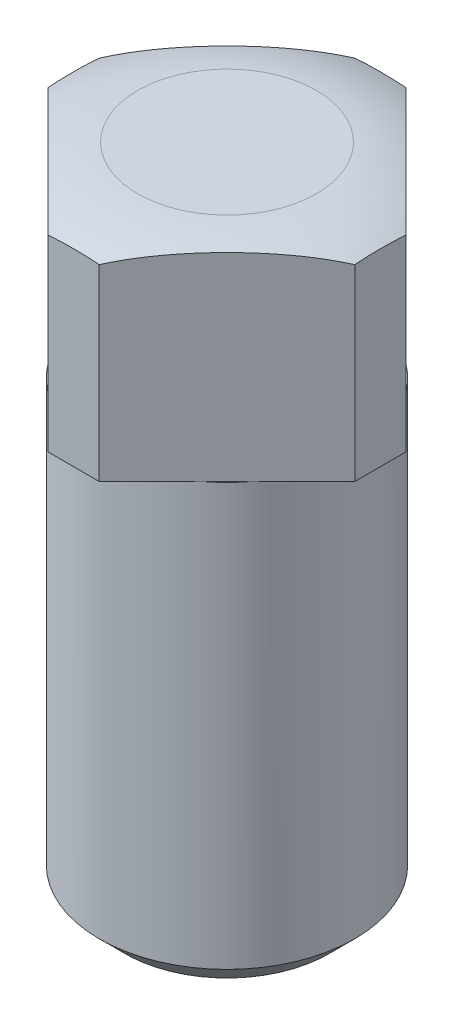
SolidWorks part; units mm, degrees
ref_plane "Front" through (0, 0, 0) normal (0, 0, 1) x (1, 0, 0)
ref_plane "Top" through (0, 0, 0) normal (0, 1, 0) x (1, 0, 0)
ref_plane "Right" through (0, 0, 0) normal (1, 0, 0) x (0, 0, -1)
sketch "Sketch1" plane through (0, 0, 0) normal (0, 0, 1) x (1, 0, 0)
  line L0 (0, 0) -> (0, 24)
  line L1 (0, 24) -> (10, 24)
  line L2 (10, 24) -> (10, 16)
  line L3 (10, 16) -> (5, 16)
  line L4 (5, 16) -> (5, 0)
  line L5 (5, 0) -> (0, 0)
  dimension "D1" = 16
  dimension "D2" = 8
  dimension "D3" = 5
  dimension "D4" = 10
revolve "Revolve1" add sketch "Sketch1" angle 360 about L0
chamfer "Chamfer1" distance 1 angle 45 1 edges at (0, 0, -5)
sketch "Sketch2" plane through (0, 24, 0) normal (0, 1, 0) x (1, 0, 0)
  line L0 (-1, 6) -> (1, 6)
  line L1 (0, 0) -> (0, 8.2576) construction
  line L2 (0, 0) -> (6, 0) construction
  line L3 (-1, -6) -> (1, -6)
  line L4 (6, 1) -> (6, -1)
  line L5 (-6, 1) -> (-6, -1)
  line L6 (-1, 6) -> (-6, 1)
  line L7 (6, 1) -> (1, 6)
  line L9 (6, -1) -> (1, -6)
  line L10 (-1, -6) -> (-6, -1)
  circle A0 centre (0, 0) radius 11.9782
  dimension "D1" = 6
  dimension "D2" = 2
  dimension "D3" = 1
  dimension "D4" = 2
  dimension "D5" = 1
  dimension "D6" = 6
extrude "Cut-Extrude2" cut sketch "Sketch2" against normal up to surface (8 mm away) up to face at (0, 16, -10)
sketch "Sketch3" plane through (0, 0, 0) normal (0, 0, 1) x (1, 0, 0)
  line L0 (3.5, 24) -> (5.5758, 25.3028)
  line L1 (5.5758, 25.3028) -> (6.4627, 23.6882)
  line L2 (3.5, 24) -> (3.5, 26.487) construction
  line L3 (6, 24) -> (1, 24) construction
  line L5 (0, 0) -> (0, 1) construction
  line L6 (-5, 1) -> (5, 1) construction
  line L7 (6.4627, 23.6882) -> (6.7583, 22.9968)
  arc A0 (3.5, 24) -> (6.7583, 22.9968) centre (3.0057, 16.6015) cw
revolve "Cut-Revolve1" cut sketch "Sketch3" angle 360 about L5
sketch "Sketch4" plane through (0, 0, 0) normal (0, -1, 0) x (1, 0, 0)
  circle A0 centre (0, 0) radius 5
extrude "Boss-Extrude1" add sketch "Sketch4" along normal mid plane 3
chamfer "Chamfer2" distance 1 angle 45 1 edges at (0, -1.5, -5)
